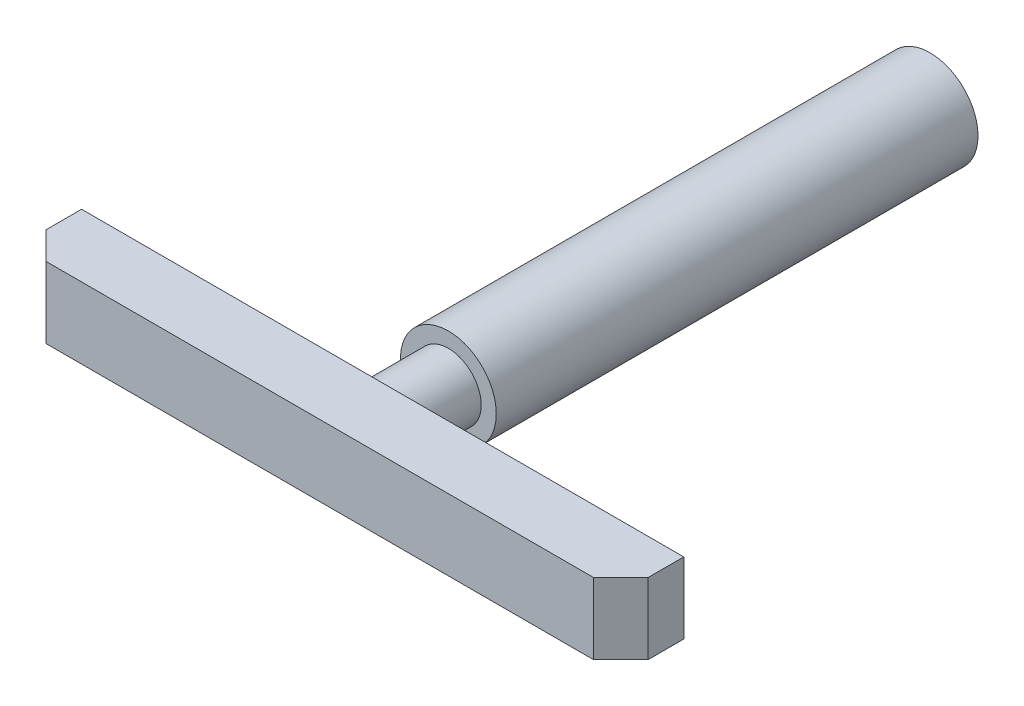
SolidWorks part; units mm, degrees
material "Q235A"
ref_plane "Front Plane" through (0, 0, 0) normal (0, 0, 1) x (1, 0, 0)
ref_plane "Top Plane" through (0, 0, 0) normal (0, 1, 0) x (1, 0, 0)
ref_plane "Right Plane" through (0, 0, 0) normal (1, 0, 0) x (0, 0, -1)
sketch "Sketch1" plane through (0, 0, 0) normal (0, 0, 1) x (1, 0, 0)
  circle A0 centre (0, 0) radius 17.5
  dimension "D1" = 35
extrude "Boss-Extrude1" add sketch "Sketch1" along normal blind 200
sketch "Sketch3" plane through (0, 0, 200) normal (0, 0, 1) x (1, 0, 0)
  circle A0 centre (0, 0) radius 12
  dimension "D1" = 24
extrude "Cut-Extrude1" cut sketch "Sketch3" against normal blind 24 flip side to cut
sketch "Sketch4" plane through (0, 0, 200) normal (0, 0, 1) x (1, 0, 0)
  line L1 (110, -13) -> (-110, -13)
  line L2 (110, -13) -> (110, 13)
  line L3 (110, 13) -> (-110, 13)
  line L4 (-110, -13) -> (-110, 13)
  line L5 (110, -13) -> (-110, 13) construction
  line L6 (110, 13) -> (-110, -13) construction
  point P0 (0, 0)
  dimension "D1" = 220
  dimension "D2" = 26
extrude "Boss-Extrude2" add sketch "Sketch4" along normal blind 23
chamfer "Chamfer1" distance 10 angle 45 2 edges at (110, 0, 223) (-110, 0, 223)
